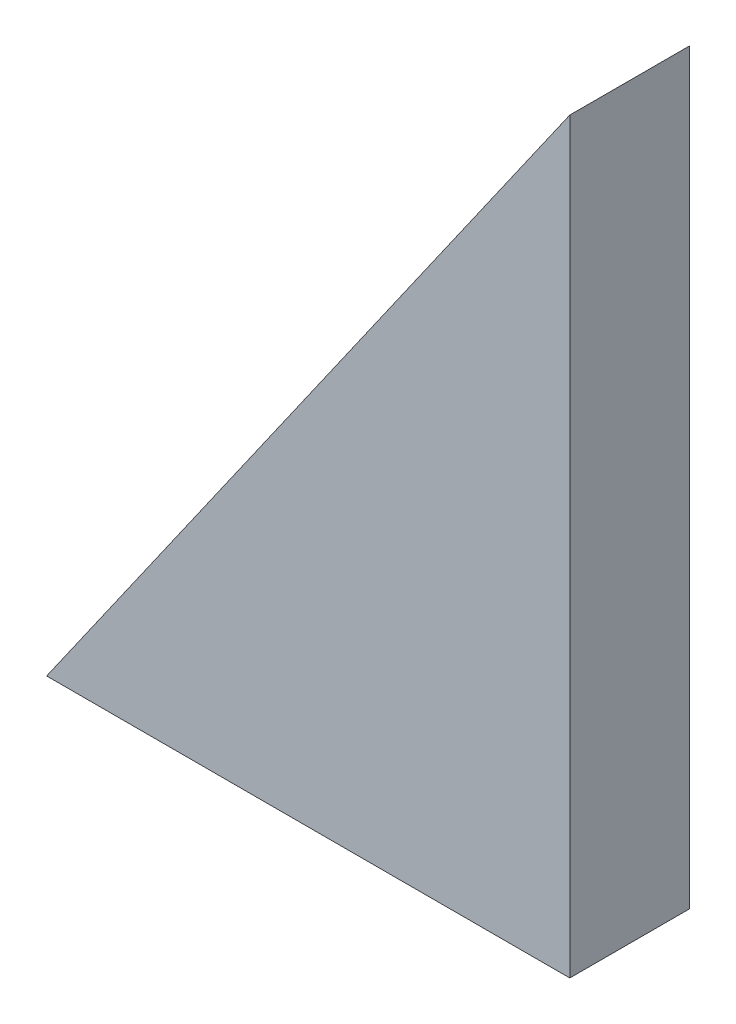
from build123d import *

# Parameters (mm, degrees)
EXTRUDE_1_DEPTH = 4


with BuildPart() as part:
    # 草图1 → 凸台-拉伸1 (new, symmetric)
    with BuildSketch(Plane.XY):
        Polygon((0, 0), (35, 0), (35, 50), align=None)
    extrude(amount=EXTRUDE_1_DEPTH, both=True)


solid = part.part
